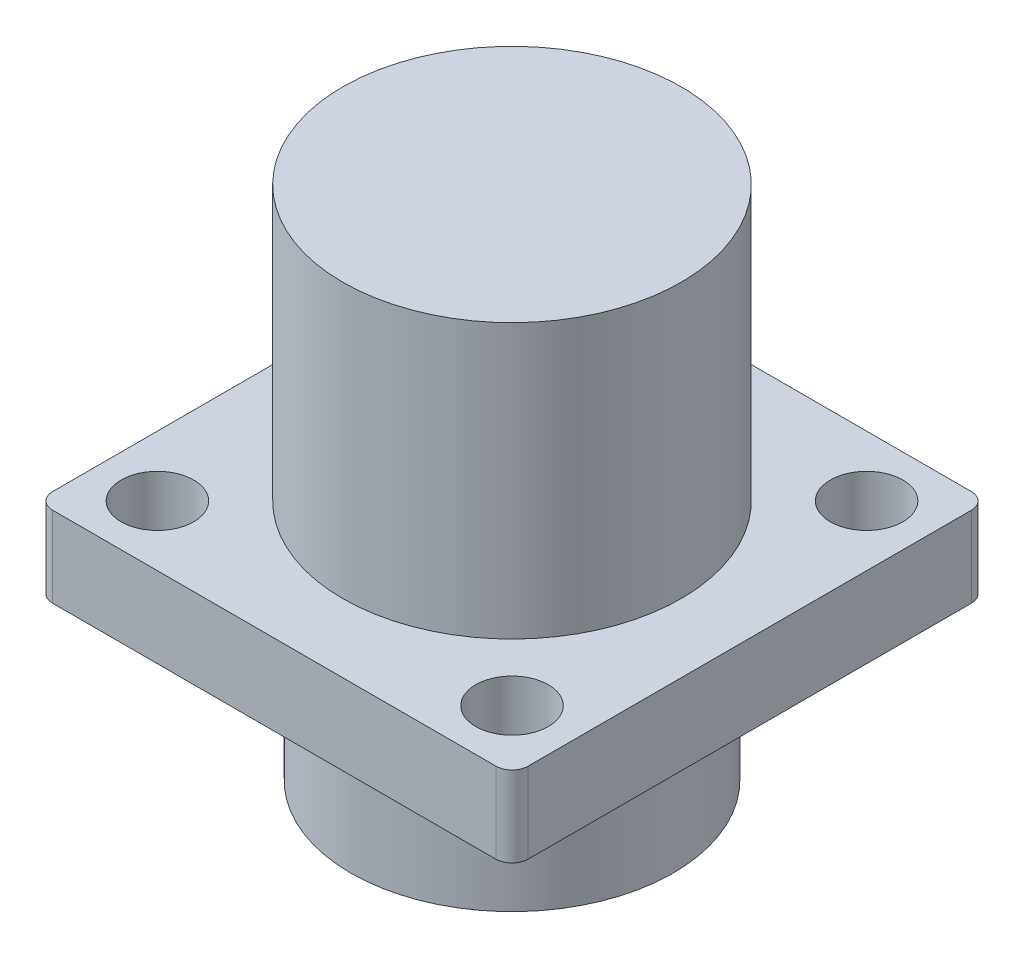
from build123d import *

# Parameters (mm, degrees)
SKETCH_1_R          = 10
EXTRUDE_1_DEPTH     = 10
SKETCH_2_W          = 29.5
SKETCH_2_H          = 29.5
EXTRUDE_2_DEPTH     = 5
SKETCH_3_R          = 10.5
EXTRUDE_3_DEPTH     = 17
SKETCH_4_R          = 2.25
CUT_EXTRUDE_1_DEPTH = 17
FILLET_1_R          = 1


with BuildPart() as part:
    # 草图1 → 凸台-拉伸1 (new body)
    with BuildSketch(Plane(origin=(0, 0, 0), x_dir=(1, 0, 0), z_dir=(0, 1, 0))):
        with Locations(Location((0, 0, 0), (0, 0, 270))):
            Circle(SKETCH_1_R)
    extrude(amount=EXTRUDE_1_DEPTH)

    # 草图2 → 凸台-拉伸2 (add)
    with BuildSketch(Plane(origin=(0, 10, 0), x_dir=(1, 0, 0), z_dir=(0, 1, 0))):
        Rectangle(SKETCH_2_W, SKETCH_2_H)
    extrude(amount=EXTRUDE_2_DEPTH)

    # 草图3 → 凸台-拉伸3 (add)
    with BuildSketch(Plane(origin=(0, 15, 0), x_dir=(1, 0, 0), z_dir=(0, 1, 0))):
        with Locations(Location((0, 0, 0), (0, 0, 270))):
            Circle(SKETCH_3_R)
    extrude(amount=EXTRUDE_3_DEPTH)

    # 草图4 → 切除-拉伸1 (cut)
    with BuildSketch(Plane(origin=(0, 15, 0), x_dir=(1, 0, 0), z_dir=(0, 1, 0))):
        with Locations(Location((11, 11, 0), (0, 0, 270))):
            Circle(SKETCH_4_R)
        with Locations(Location((-11, 11, 0), (0, 0, 270))):
            Circle(SKETCH_4_R)
        with Locations(Location((-11, -11, 0), (0, 0, 270))):
            Circle(SKETCH_4_R)
        with Locations(Location((11, -11, 0), (0, 0, 270))):
            Circle(SKETCH_4_R)
    extrude(amount=-CUT_EXTRUDE_1_DEPTH, mode=Mode.SUBTRACT)

    # 圆角1
    fillet_1_edges = [part.edges().sort_by_distance(p)[0] for p in [
        (14.75, 12.5, 14.75),
        (14.75, 12.5, -14.75),
        (-14.75, 12.5, -14.75),
        (-14.75, 12.5, 14.75),
    ]]
    fillet(fillet_1_edges, radius=FILLET_1_R)


solid = part.part
